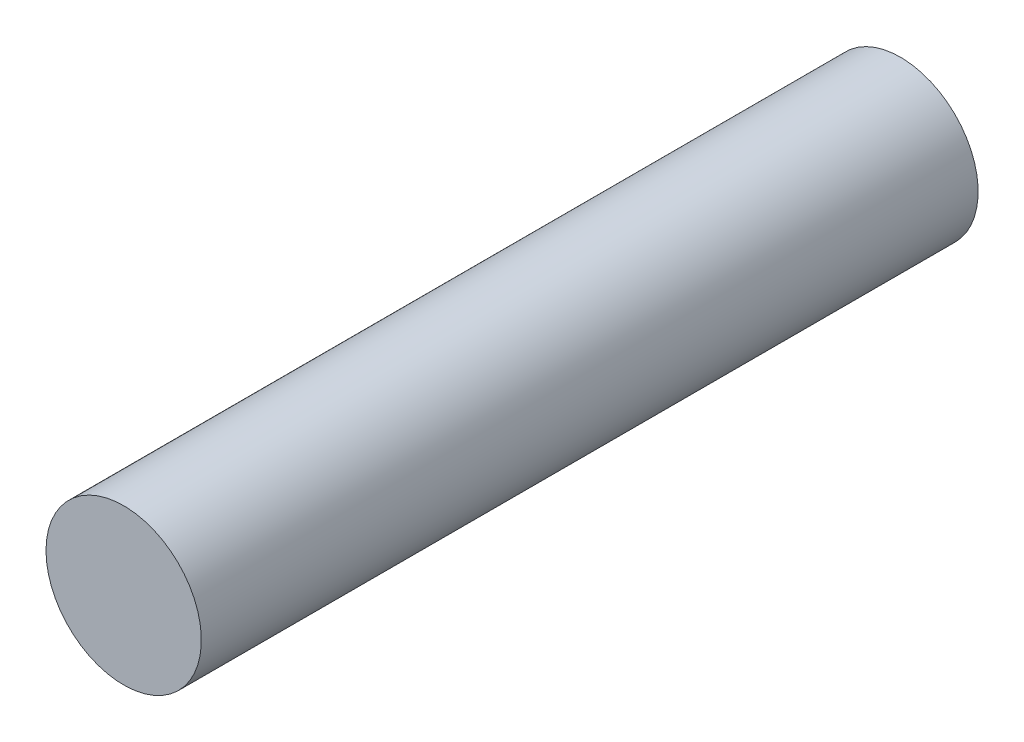
from build123d import *

# Parameters (mm, degrees)
SKETCH1_W = 7.5
SKETCH1_H = 75


with BuildPart() as part:
    # Sketch1 → Revolve1 (revolve)
    with BuildSketch(Plane.XZ, mode=Mode.PRIVATE) as revolve1_sk:
        with Locations((3.75, 37.5)):
            Rectangle(SKETCH1_W, SKETCH1_H)
    revolve(revolve1_sk.sketch.rotate(Axis((0, 0, 75), (0, 0, -1)), 180), axis=Axis((0, 0, 75), (0, 0, -1)))


solid = part.part
